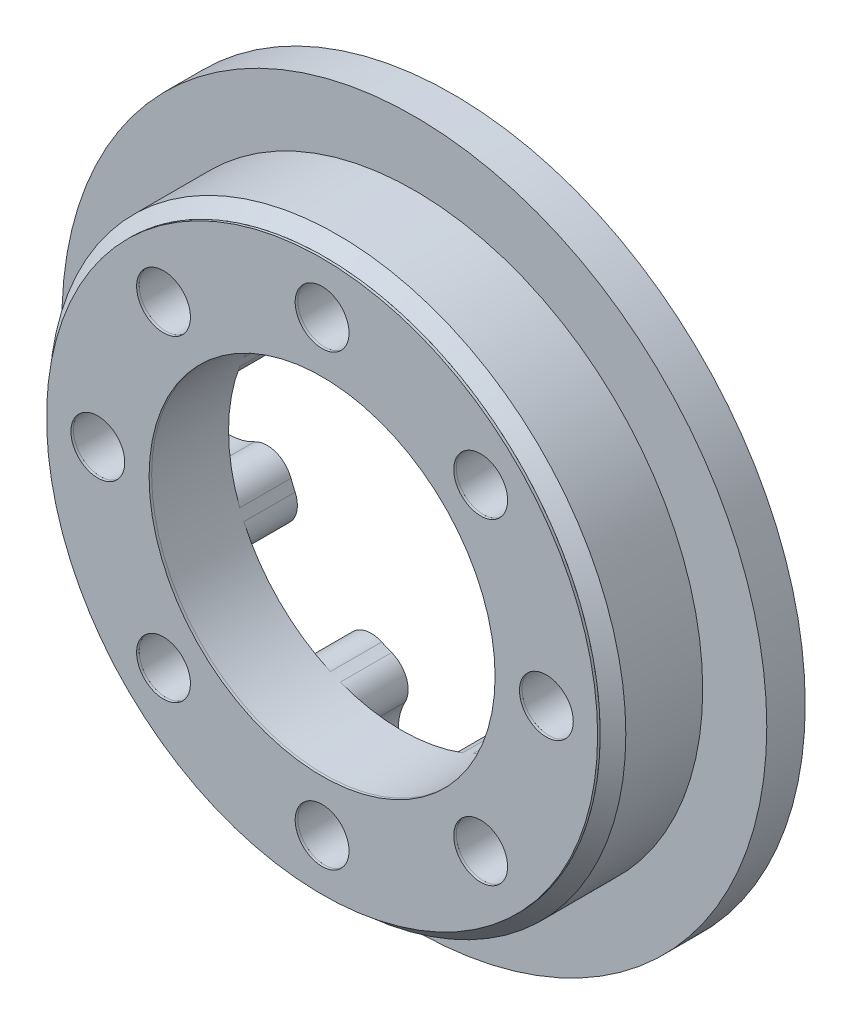
from build123d import *

# Parameters (mm, degrees)
SKETCH_2_R          = 2.1
CUT_EXTRUDE_1_DEPTH = 41.155946011
SKETCH_3_R          = 4.25
CUT_EXTRUDE_5_DEPTH = 4
FILLET_1_R          = 2
CHAMFER_2_SIZE      = 1
SKETCH_4_R          = 21.5
SKETCH_4_R_2        = 13.5
SKETCH_4_R_3        = 2.1
EXTRUDE_1_DEPTH     = 0.2


with BuildPart() as part:
    # 草图1 → 旋转1 (revolve)
    with BuildSketch(Plane(origin=(0, 0, 0), x_dir=(1, 0, 0), z_dir=(0, 1, 0)), mode=Mode.PRIVATE) as revolve_1_sk:
        Polygon((-27.5, 10), (-27.5, 7), (-22.5, 7), (-22.5, 0), (-13.5, 0), (-13.5, 10), align=None)
    revolve(revolve_1_sk.sketch.rotate(Axis((0, 0, 386.502260242), (0, 0, -1)), 180), axis=Axis((0, 0, 386.502260242), (0, 0, -1)))

    # 草图2 → 切除-拉伸1 (cut, through all)
    with BuildSketch(Plane(origin=(0, 0, -10), x_dir=(-1, 0, 0), z_dir=(0, 0, -1))):
        with Locations((0, 17.5)):
            Circle(SKETCH_2_R)
        with Locations((12.374368671, 12.374368671)):
            Circle(SKETCH_2_R)
        with Locations((17.5, 0)):
            Circle(SKETCH_2_R)
        with Locations((12.374368671, -12.374368671)):
            Circle(SKETCH_2_R)
        with Locations((0, -17.5)):
            Circle(SKETCH_2_R)
        with Locations((-12.374368671, -12.374368671)):
            Circle(SKETCH_2_R)
        with Locations((-17.5, 0)):
            Circle(SKETCH_2_R)
        with Locations((-12.374368671, 12.374368671)):
            Circle(SKETCH_2_R)
    extrude(amount=-CUT_EXTRUDE_1_DEPTH, mode=Mode.SUBTRACT)

    # 草图3 → 切除-拉伸5 (cut)
    with BuildSketch(Plane(origin=(0, 0, -10), x_dir=(-1, 0, 0), z_dir=(0, 0, -1))):
        with Locations((0, 17.5)):
            Circle(SKETCH_3_R)
        with Locations((12.374368671, 12.374368671)):
            Circle(SKETCH_3_R)
        with Locations((17.5, 0)):
            Circle(SKETCH_3_R)
        with Locations((12.374368671, -12.374368671)):
            Circle(SKETCH_3_R)
        with Locations((0, -17.5)):
            Circle(SKETCH_3_R)
        with Locations((-12.374368671, -12.374368671)):
            Circle(SKETCH_3_R)
        with Locations((-17.5, 0)):
            Circle(SKETCH_3_R)
        with Locations((-12.374368671, 12.374368671)):
            Circle(SKETCH_3_R)
    extrude(amount=-CUT_EXTRUDE_5_DEPTH, mode=Mode.SUBTRACT)

    # 圆角1
    fillet_1_edges = [part.edges().sort_by_distance(p)[0] for p in [
        (1.259999544, 13.441071429, -8),
        (-1.259999544, 13.441071429, -8),
        (-8.613318531, 10.395226976, -8),
        (-10.395226976, 8.613318531, -8),
        (-13.441071429, 1.259999544, -8),
        (-13.441071429, -1.259999544, -8),
        (-10.395226976, -8.613318531, -8),
        (-8.613318531, -10.395226976, -8),
        (-1.259999544, -13.441071429, -8),
        (1.259999544, -13.441071429, -8),
        (8.613318531, -10.395226976, -8),
        (10.395226976, -8.613318531, -8),
        (13.441071429, -1.259999544, -8),
        (13.441071429, 1.259999544, -8),
        (10.395226976, 8.613318531, -8),
        (8.613318531, 10.395226976, -8),
    ]]
    fillet(fillet_1_edges, radius=FILLET_1_R)

    # 倒角2
    chamfer_2_edges = [part.edges().sort_by_distance(p)[0] for p in [
        (-22.5, 0, 0),
    ]]
    chamfer(chamfer_2_edges, length=CHAMFER_2_SIZE)


with BuildPart() as body_2:
    # 草图4 → 凸台-拉伸1 (new body)
    with BuildSketch(Plane.XY):
        Circle(SKETCH_4_R)
        Circle(SKETCH_4_R_2, mode=Mode.SUBTRACT)
        with Locations((-12.374368671, 12.374368671)):
            Circle(SKETCH_4_R_3, mode=Mode.SUBTRACT)
        with Locations((-17.5, 0)):
            Circle(SKETCH_4_R_3, mode=Mode.SUBTRACT)
        with Locations((-12.374368671, -12.374368671)):
            Circle(SKETCH_4_R_3, mode=Mode.SUBTRACT)
        with Locations((0, -17.5)):
            Circle(SKETCH_4_R_3, mode=Mode.SUBTRACT)
        with Locations((12.374368671, -12.374368671)):
            Circle(SKETCH_4_R_3, mode=Mode.SUBTRACT)
        with Locations((17.5, 0)):
            Circle(SKETCH_4_R_3, mode=Mode.SUBTRACT)
        with Locations((12.374368671, 12.374368671)):
            Circle(SKETCH_4_R_3, mode=Mode.SUBTRACT)
        with Locations((0, 17.5)):
            Circle(SKETCH_4_R_3, mode=Mode.SUBTRACT)
    extrude(amount=EXTRUDE_1_DEPTH)


solid = Compound([part.part, body_2.part])
